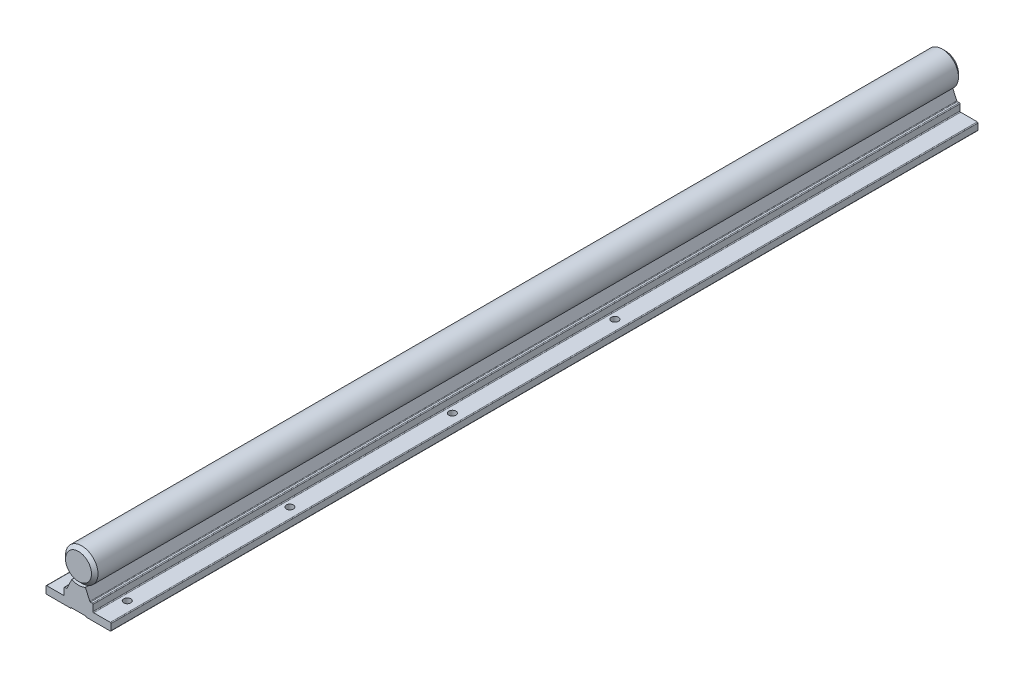
from build123d import *

# Parameters (mm, degrees)
SKETCH6_R                      = 15
BOSS_EXTRUDE2_DEPTH            = 800
CHAMFER1_SIZE                  = 3
BOSS_EXTRUDE1_DEPTH            = 800
SKETCH4_W                      = 3.3
SKETCH4_H                      = 7
CURVE_PATTERN1_COUNT           = 4
CURVE_PATTERN1_PITCH           = 150
CURVE_PATTERN1_COPY_1_SKETCH_W = 3.3
CURVE_PATTERN1_COPY_1_SKETCH_H = 7
CURVE_PATTERN1_COPY_2_SKETCH_W = 3.3
CURVE_PATTERN1_COPY_2_SKETCH_H = 7
CURVE_PATTERN1_COPY_3_SKETCH_W = 3.3
CURVE_PATTERN1_COPY_3_SKETCH_H = 7


with BuildPart() as part:
    # Sketch6 → Boss-Extrude2 (new body)
    with BuildSketch(Plane.XY):
        with Locations((0, 37)):
            Circle(SKETCH6_R)
    extrude(amount=-BOSS_EXTRUDE2_DEPTH)

    # Chamfer1
    chamfer1_edges = [part.edges().sort_by_distance(p)[0] for p in [
        (-15, 37, 0),
        (-15, 37, -800),
    ]]
    chamfer(chamfer1_edges, length=CHAMFER1_SIZE)

    # Sketch3 → Boss-Extrude1 (add)
    with BuildSketch(Plane.XY):
        with BuildLine():
            Line((-10.499533732, 14.404167217), (-6.30880391, 23.391216321))
            ThreePointArc((-6.30880391, 23.391216321), (0, 22), (6.30880391, 23.391216321))
            Line((6.30880391, 23.391216321), (10.499533732, 14.404167217))
            ThreePointArc((10.499533732, 14.404167217), (10.757839457, 14.109625988), (11.133949183, 14))
            Line((11.133949183, 14), (12.66, 14))
            ThreePointArc((12.66, 14), (13.154974747, 13.794974747), (13.36, 13.3))
            Line((13.36, 13.3), (13.36, 7.7))
            ThreePointArc((13.36, 7.7), (13.565025253, 7.205025253), (14.06, 7))
            Line((14.06, 7), (29.3, 7))
            ThreePointArc((29.3, 7), (29.794974747, 6.794974747), (30, 6.3))
            Line((30, 6.3), (30, 0.7))
            ThreePointArc((30, 0.7), (29.794974747, 0.205025253), (29.3, 0))
            Line((29.3, 0), (7, 0))
            Line((7, 0), (7, 0.7))
            Line((7, 0.7), (-7, 0.7))
            Line((-7, 0.7), (-7, 0))
            Line((-7, 0), (-29.3, 0))
            ThreePointArc((-29.3, 0), (-29.794974747, 0.205025253), (-30, 0.7))
            Line((-30, 0.7), (-30, 6.3))
            ThreePointArc((-30, 6.3), (-29.794974747, 6.794974747), (-29.3, 7))
            Line((-29.3, 7), (-14.06, 7))
            ThreePointArc((-14.06, 7), (-13.565025253, 7.205025253), (-13.36, 7.7))
            Line((-13.36, 7.7), (-13.36, 13.3))
            ThreePointArc((-13.36, 13.3), (-13.154974747, 13.794974747), (-12.66, 14))
            Line((-12.66, 14), (-11.133949183, 14))
            ThreePointArc((-11.133949183, 14), (-10.757839457, 14.109625988), (-10.499533732, 14.404167217))
        make_face()
    extrude(amount=-BOSS_EXTRUDE1_DEPTH)

    # Sketch4 → Cut-Revolve1 (revolve, cut)
    with BuildSketch(Plane.XY.offset(-25), mode=Mode.PRIVATE) as cut_revolve1_sk:
        with Locations((-21.65, 3.5)):
            Rectangle(SKETCH4_W, SKETCH4_H)
    cut_revolve1 = revolve(cut_revolve1_sk.sketch.rotate(Axis((-20, 7, -25), (0, -1, 0)), 270), axis=Axis((-20, 7, -25), (0, -1, 0)), mode=Mode.SUBTRACT)

    # Mirror1: Cut-Revolve1 across plane
    add(cut_revolve1.mirror(Plane(origin=(0, 0, 0), x_dir=(0, 0, 1), z_dir=(1, 0, 0))), mode=Mode.SUBTRACT)

    # Sketch5 → Cut-Revolve2 (revolve, cut)
    with BuildSketch(Plane.XY.offset(-25)):
        Polygon((-7, 0.7), (-7, 9.1), (-2.8, 9.1), (-2.8, 34.475681392), (0, 34.475681392), (0, 0.7), align=None)
    cut_revolve2 = revolve(axis=Axis((0, 34.475681392, -25), (0, -1, 0)), mode=Mode.SUBTRACT)

    # Curve Pattern1: Cut-Revolve1, Cut-Revolve2 ×4
    with Locations(*[(0, 0, -i * CURVE_PATTERN1_PITCH) for i in range(1, CURVE_PATTERN1_COUNT)]):
        add(cut_revolve1, mode=Mode.SUBTRACT)
        add(cut_revolve2, mode=Mode.SUBTRACT)

    # Curve Pattern1 copy 1 sketch → Curve Pattern1 copy 1 (revolve, cut)
    with BuildSketch(Plane(origin=(0, 0, -175), x_dir=(-1, 0, 0), z_dir=(0, 0, 1))):
        with Locations((-21.65, -3.5)):
            Rectangle(CURVE_PATTERN1_COPY_1_SKETCH_W, CURVE_PATTERN1_COPY_1_SKETCH_H)
    revolve(axis=Axis((20, 7, -175), (0, 1, 0)), mode=Mode.SUBTRACT)

    # Curve Pattern1 copy 2 sketch → Curve Pattern1 copy 2 (revolve, cut)
    with BuildSketch(Plane(origin=(0, 0, -325), x_dir=(-1, 0, 0), z_dir=(0, 0, 1))):
        with Locations((-21.65, -3.5)):
            Rectangle(CURVE_PATTERN1_COPY_2_SKETCH_W, CURVE_PATTERN1_COPY_2_SKETCH_H)
    revolve(axis=Axis((20, 7, -325), (0, 1, 0)), mode=Mode.SUBTRACT)

    # Curve Pattern1 copy 3 sketch → Curve Pattern1 copy 3 (revolve, cut)
    with BuildSketch(Plane(origin=(0, 0, -475), x_dir=(-1, 0, 0), z_dir=(0, 0, 1))):
        with Locations((-21.65, -3.5)):
            Rectangle(CURVE_PATTERN1_COPY_3_SKETCH_W, CURVE_PATTERN1_COPY_3_SKETCH_H)
    revolve(axis=Axis((20, 7, -475), (0, 1, 0)), mode=Mode.SUBTRACT)


solid = part.part
